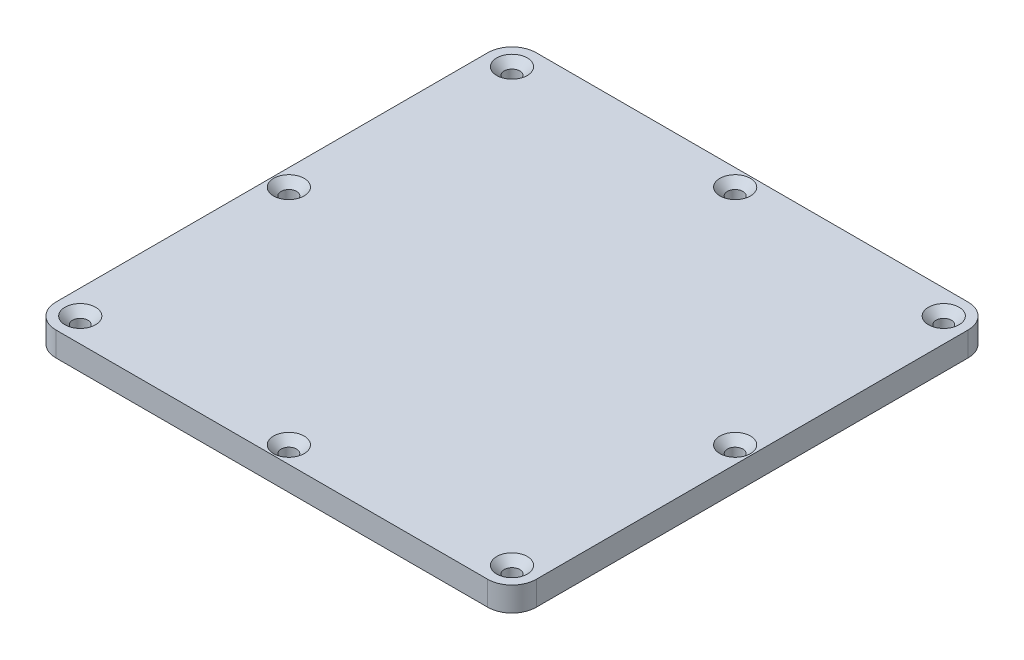
SolidWorks part; units mm, degrees
ref_plane "Front Plane" through (0, 0, 0) normal (0, 0, 1) x (1, 0, 0)
ref_plane "Top Plane" through (0, 0, 0) normal (0, 1, 0) x (1, 0, 0)
ref_plane "Right Plane" through (0, 0, 0) normal (1, 0, 0) x (0, 0, -1)
sketch "Sketch1" plane through (0, 0, 0) normal (0, 1, 0) x (1, 0, 0)
  line L1 (-49.5, -49.5) -> (49.5, -49.5)
  line L2 (-49.5, -49.5) -> (-49.5, 49.5)
  line L3 (-49.5, 49.5) -> (49.5, 49.5)
  line L4 (49.5, -49.5) -> (49.5, 49.5)
  line L5 (-49.5, -49.5) -> (49.5, 49.5) construction
  line L6 (-49.5, 49.5) -> (49.5, -49.5) construction
  point P0 (0, 0)
  dimension "D1" = 99
  dimension "D2" = 99
extrude "Boss-Extrude1" add sketch "Sketch1" along normal blind 5
fillet "Fillet1" radius 5 4 edges at (-49.5, 2.5, 49.5) (49.5, 2.5, 49.5) (49.5, 2.5, -49.5) (-49.5, 2.5, -49.5)
hole_wizard "CSK for M3 Flat Head Machine Screw1" positions "Sketch2" profile "Sketch3" countersink size "M3" standard "ANSI Metric"
sketch "Sketch2" plane through (0, 5, 0) normal (0, 1, 0) x (1, 0, 0)
  line L0 (44.5, 49.5) -> (-44.5, 49.5) construction
  line L1 (49.5, -44.5) -> (49.5, 44.5) construction
  line L2 (-49.5, 44.5) -> (-49.5, -44.5) construction
  line L3 (-44.5, -49.5) -> (44.5, -49.5) construction
  point P0 (-44.5, 44.5)
  point P2 (44.5, 44.5)
  point P4 (0, 46)
  point P6 (-46, 0)
  point P8 (-44.5, -44.5)
  point P10 (0, -46)
  point P12 (44.5, -44.5)
  point P14 (46, 0)
  dimension "D1" = 3.5
  dimension "D2" = 5
  dimension "D3" = 5
  dimension "D4" = 5
  dimension "D5" = 5
  dimension "D6" = 49.5
  dimension "D7" = 3.5
  dimension "D8" = 5
  dimension "D9" = 5
  dimension "D10" = 49.5
  dimension "D11" = 3.5
  dimension "D12" = 49.5
  dimension "D13" = 5
  dimension "D14" = 5
  dimension "D15" = 3.5
  dimension "D16" = 49.5
sketch "Sketch3" plane through (-44.5, 5, -44.5) normal (1, 0, 0) x (0, 0, 1)
  line L0 (0, 0) -> (0, 9.4614)
  line L1 (0, 9.4614) -> (1.6, 8.5)
  line L2 (1.6, 8.5) -> (1.6, 1.55)
  line L3 (1.6, 1.55) -> (3.15, 0)
  line L5 (3.15, 0) -> (0, 0)
  line L6 (-1.6, 1.55) -> (-3.15, 0) construction
  line L10 (0, 9.4614) -> (-1.6, 8.5) construction
  line L11 (0, -6.35) -> (0, 107.95) construction
  dimension "孔直径" = 3.2
  dimension "孔深度" = 8.5
  dimension "近端锥形沉头孔直径" = 6.3
  dimension "近端锥形沉头孔角度" = 90
  dimension "导头角度" = 118
sketch "Sketch4" plane through (0, 0, 0) normal (0, -1, 0) x (1, 0, 0)
  line L1 (39.5, 35) -> (-39.5, 35)
  line L2 (39.5, 35) -> (39.5, -35)
  line L3 (39.5, -35) -> (-39.5, -35)
  line L4 (-39.5, 35) -> (-39.5, -35)
  line L5 (39.5, 35) -> (-39.5, -35) construction
  line L6 (39.5, -35) -> (-39.5, 35) construction
  point P0 (0, 0)
  dimension "D1" = 79
  dimension "D2" = 70
